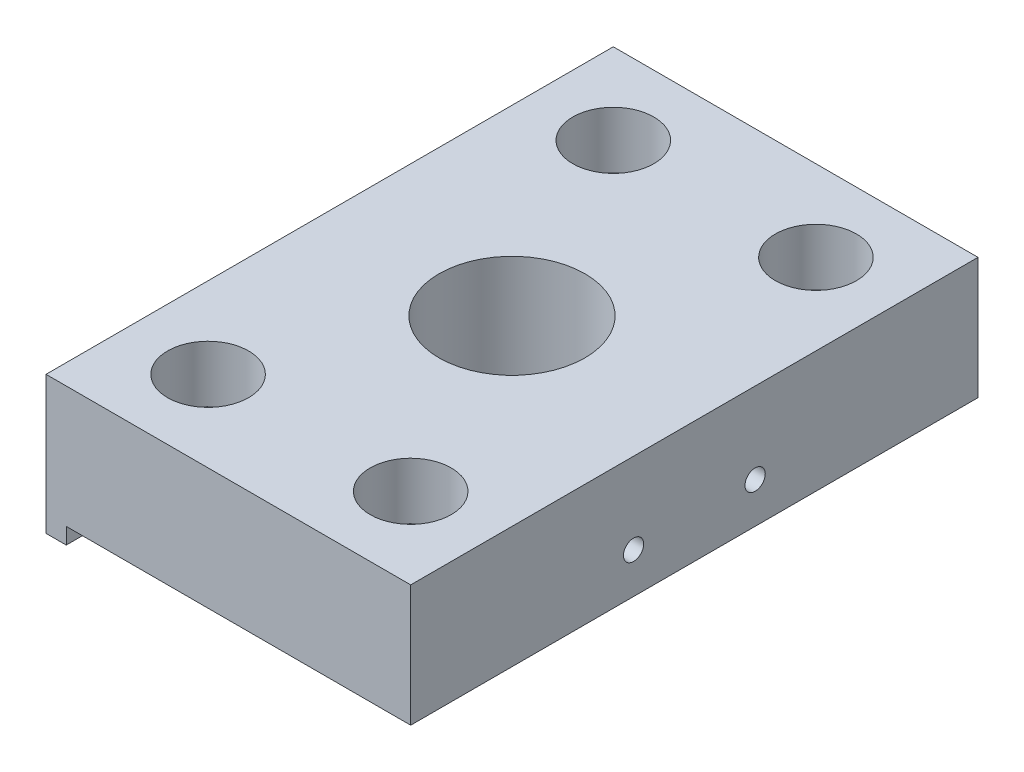
from build123d import *

# Parameters (mm, degrees)
SKETCH_1_W                = 45
SKETCH_1_H                = 70
EXTRUDE_1_DEPTH           = 8.5
SKETCH_2_W                = 42.5
SKETCH_2_H                = 70
CUT_EXTRUDE_1_DEPTH       = 2
HOLE_WIZARD_1_D           = 5.5
HOLE_WIZARD_1_CBORE_D     = 10
HOLE_WIZARD_1_CBORE_DEPTH = 7
HOLE_WIZARD_18_0_18_1_D   = 18
HOLE_WIZARD_M3_1_D        = 2.5
HOLE_WIZARD_M3_1_DEPTH    = 8.5
HOLE_WIZARD_M3_1_TIP      = 0.751075774


with BuildPart() as part:
    # 草图1 → 凸台-拉伸1 (new, symmetric)
    with BuildSketch(Plane(origin=(0, 0, 0), x_dir=(1, 0, 0), z_dir=(0, 1, 0))):
        Rectangle(SKETCH_1_W, SKETCH_1_H)
    extrude(amount=EXTRUDE_1_DEPTH, both=True)

    # 草图2 → 切除-拉伸1 (cut)
    with BuildSketch(Plane.XZ.offset(8.5)):
        with Locations((1.25, 0)):
            Rectangle(SKETCH_2_W, SKETCH_2_H)
    extrude(amount=-CUT_EXTRUDE_1_DEPTH, mode=Mode.SUBTRACT)

    # 打孔尺寸(%根据)内六角圆柱头螺钉的类型1 (through all)
    with Locations(Plane(origin=(0, 8.5, 0), x_dir=(1, 0, 0), z_dir=(0, 1, 0))):
        with Locations((-12.5, -25), (-12.5, 25), (12.5, 25), (12.5, -25)):
            CounterBoreHole(HOLE_WIZARD_1_D / 2, HOLE_WIZARD_1_CBORE_D / 2, HOLE_WIZARD_1_CBORE_DEPTH)

    # Ø18.0 (18) 直径孔1 (through all)
    with Locations(Plane(origin=(0, 8.5, 0), x_dir=(1, 0, 0), z_dir=(0, 1, 0))):
        with Locations((0, 0)):
            Hole(HOLE_WIZARD_18_0_18_1_D / 2)

    # M3 螺纹孔1
    with Locations(Plane(origin=(22.5, 0, 0), x_dir=(0, 0, -1), z_dir=(1, 0, 0))):
        with Locations((7.5, -1.5), (-7.5, -1.5)):
            Hole(HOLE_WIZARD_M3_1_D / 2, depth=HOLE_WIZARD_M3_1_DEPTH)
            with Locations((0, 0, -(HOLE_WIZARD_M3_1_DEPTH + HOLE_WIZARD_M3_1_TIP / 2))):  # 118° drill point
                Cone(0, HOLE_WIZARD_M3_1_D / 2, HOLE_WIZARD_M3_1_TIP, mode=Mode.SUBTRACT)


solid = part.part
